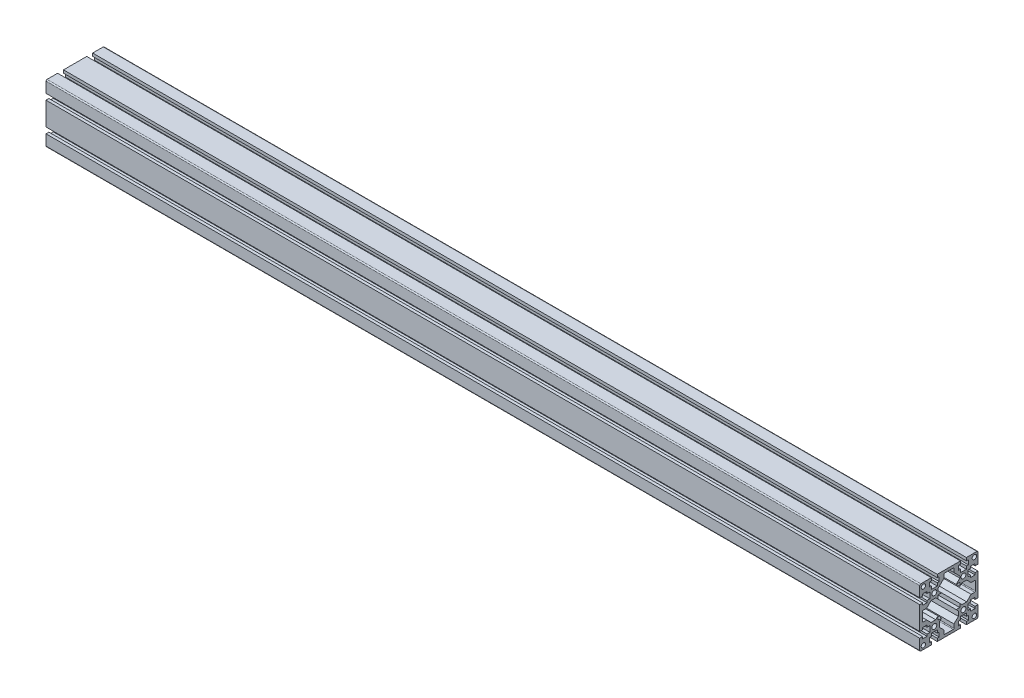
SolidWorks part; units mm, degrees
ref_plane "Front Plane" through (0, 0, 0) normal (0, 0, 1) x (1, 0, 0)
ref_plane "Top Plane" through (0, 0, 0) normal (0, 1, 0) x (1, 0, 0)
ref_plane "Right Plane" through (0, 0, 0) normal (1, 0, 0) x (0, 0, -1)
sketch "草图1" plane through (0, 0, 0) normal (0, 0, 1) x (1, 0, 0)
  line L0 (-530.3448, 0) -> (669.6552, 0)
  dimension "D1" = 1200
other "Aluminium profile 80 X 80G X R1.5(1)"
ref_plane "Plane2" through (-530.3448, 0, 0) normal (1, 0, 0) x (0, 1, 0)
sketch "Sketch1" plane through (-530.3448, 0, 0) normal (1, 0, 0) x (0, 1, 0)
  line L0 (0, 40) -> (0, 0) construction
  line L1 (0, 0) -> (40, 0) construction
  line L2 (-24.05, 40) -> (-24.05, 36)
  line L3 (-38.5, 40) -> (-24.05, 40)
  line L4 (-40, 38.5) -> (-40, 24.05)
  line L5 (-38.5, -40) -> (-24.05, -40)
  line L6 (40, 38.5) -> (40, 24.05)
  line L7 (-24.05, 36) -> (-26.75, 36)
  line L8 (-26.75, 36) -> (-26.75, 30)
  line L9 (-26.75, 30) -> (-24.05, 30)
  line L10 (-24.05, 30) -> (-24.05, 26)
  line L11 (-24.05, 26) -> (-15.95, 26)
  line L12 (-15.95, 26) -> (-15.95, 30)
  line L13 (-15.95, 30) -> (-13.25, 30)
  line L14 (-13.25, 30) -> (-13.25, 36)
  line L15 (-13.25, 36) -> (-15.95, 36)
  line L16 (-15.95, 36) -> (-15.95, 40)
  line L17 (-40, 15.95) -> (-36, 15.95)
  line L18 (-36, 15.95) -> (-36, 13.25)
  line L19 (-15.95, 40) -> (15.95, 40)
  line L20 (-20, 20) -> (-20, 40) construction
  line L21 (20, 20) -> (20, 40) construction
  line L22 (15.95, 36) -> (15.95, 40)
  line L23 (13.25, 36) -> (15.95, 36)
  line L24 (13.25, 30) -> (13.25, 36)
  line L25 (15.95, 30) -> (13.25, 30)
  line L26 (-36, 13.25) -> (-30, 13.25)
  line L27 (-30, 13.25) -> (-30, 15.95)
  line L28 (-26, 15.95) -> (-26, 24.05)
  line L29 (-26, 24.05) -> (-30, 24.05)
  line L30 (-30, 24.05) -> (-30, 26.75)
  line L31 (-30, 26.75) -> (-36, 26.75)
  line L32 (-36, 26.75) -> (-36, 24.05)
  line L33 (-36, 24.05) -> (-40, 24.05)
  line L34 (-30, 15.95) -> (-26, 15.95)
  line L35 (15.95, 26) -> (15.95, 30)
  line L36 (24.05, 26) -> (15.95, 26)
  line L37 (24.05, 30) -> (24.05, 26)
  line L38 (26.75, 30) -> (24.05, 30)
  line L39 (26.75, 36) -> (26.75, 30)
  line L40 (24.05, 36) -> (26.75, 36)
  line L41 (24.05, 40) -> (24.05, 36)
  line L42 (24.05, -40) -> (24.05, -36)
  line L43 (24.05, -36) -> (26.75, -36)
  line L44 (26.75, -36) -> (26.75, -30)
  line L45 (26.75, -30) -> (24.05, -30)
  line L46 (24.05, -30) -> (24.05, -26)
  line L47 (24.05, -26) -> (15.95, -26)
  line L48 (15.95, -26) -> (15.95, -30)
  line L49 (15.95, -30) -> (13.25, -30)
  line L50 (13.25, -30) -> (13.25, -36)
  line L51 (13.25, -36) -> (15.95, -36)
  line L52 (15.95, -36) -> (15.95, -40)
  line L53 (-15.95, -36) -> (-15.95, -40)
  line L54 (-13.25, -36) -> (-15.95, -36)
  line L55 (-13.25, -30) -> (-13.25, -36)
  line L56 (-15.95, -30) -> (-13.25, -30)
  line L57 (-15.95, -26) -> (-15.95, -30)
  line L58 (-24.05, -26) -> (-15.95, -26)
  line L59 (-24.05, -30) -> (-24.05, -26)
  line L60 (-26.75, -30) -> (-24.05, -30)
  line L61 (-26.75, -36) -> (-26.75, -30)
  line L62 (-24.05, -36) -> (-26.75, -36)
  line L63 (-24.05, -40) -> (-24.05, -36)
  line L64 (-30, -15.95) -> (-26, -15.95)
  line L65 (-36, -26.75) -> (-36, -24.05)
  line L66 (-30, -26.75) -> (-36, -26.75)
  line L67 (-30, -24.05) -> (-30, -26.75)
  line L68 (-26, -24.05) -> (-30, -24.05)
  line L69 (-26, -15.95) -> (-26, -24.05)
  line L70 (-30, -13.25) -> (-30, -15.95)
  line L71 (-36, -13.25) -> (-30, -13.25)
  line L72 (-36, -15.95) -> (-36, -13.25)
  line L73 (36, 24.05) -> (40, 24.05)
  line L74 (40, 15.95) -> (36, 15.95)
  line L75 (36, -15.95) -> (36, -13.25)
  line L76 (36, -13.25) -> (30, -13.25)
  line L77 (30, -13.25) -> (30, -15.95)
  line L78 (26, -15.95) -> (26, -24.05)
  line L79 (26, -24.05) -> (30, -24.05)
  line L80 (30, -24.05) -> (30, -26.75)
  line L81 (30, -26.75) -> (36, -26.75)
  line L82 (36, -26.75) -> (36, -24.05)
  line L83 (30, -15.95) -> (26, -15.95)
  line L84 (30, 15.95) -> (26, 15.95)
  line L85 (36, 26.75) -> (36, 24.05)
  line L86 (30, 26.75) -> (36, 26.75)
  line L87 (30, 24.05) -> (30, 26.75)
  line L88 (26, 24.05) -> (30, 24.05)
  line L89 (26, 15.95) -> (26, 24.05)
  line L90 (30, 13.25) -> (30, 15.95)
  line L91 (36, 13.25) -> (30, 13.25)
  line L92 (36, 15.95) -> (36, 13.25)
  line L93 (-36, -15.95) -> (-40, -15.95)
  line L94 (-36, -24.05) -> (-40, -24.05)
  line L95 (36, -15.95) -> (40, -15.95)
  line L96 (36, -24.05) -> (40, -24.05)
  line L97 (-13, 18) -> (-10, 15)
  line L98 (-15, 15) -> (-10, 15)
  line L99 (-15, 15) -> (-15, 10)
  line L100 (-15, -15) -> (-10, -15)
  line L101 (15, 15) -> (15, 10)
  line L102 (-18, 13) -> (-15, 10)
  line L104 (13, 18) -> (10, 15)
  line L105 (13, -18) -> (10, -15)
  line L106 (20, -15) -> (15, -10)
  line L107 (-18, -13) -> (-15, -10)
  line L108 (-13, -18) -> (-10, -15)
  line L109 (15, -10) -> (15, -15)
  line L110 (10, 15) -> (15, 15)
  line L111 (-15, -10) -> (-15, -15)
  line L112 (10, -15) -> (15, -15)
  line L113 (15, 10) -> (20, 15)
  line L235 (24.05, 40) -> (38.5, 40)
  line L249 (-40, 15.95) -> (-40, -15.95)
  line L250 (-20, 20) -> (-26, 20) construction
  line L264 (40, 15.95) -> (40, -15.95)
  line L265 (-13, 24.5) -> (-7, 30.5)
  line L266 (-7, 30.5) -> (-7, 35.5)
  line L267 (7, 35.5) -> (7, 30.5)
  line L268 (7, 30.5) -> (13, 24.5)
  line L269 (-6, -36.5) -> (6, -36.5)
  line L270 (-13, 24.5) -> (-13, 18)
  line L271 (-35.5, 7) -> (-30.5, 7)
  line L272 (-30.5, 7) -> (-24.5, 13)
  line L273 (-24.5, 13) -> (-18, 13)
  line L274 (13, 24.5) -> (13, 18)
  line L275 (-15.95, -40) -> (15.95, -40)
  line L276 (35.5, 7) -> (30.5, 7)
  line L277 (30.5, 7) -> (22.5, 15)
  line L278 (24.05, -40) -> (38.5, -40)
  line L279 (20, 15) -> (22.5, 15)
  line L333 (-13, -24.5) -> (-13, -18)
  line L336 (-13, -24.5) -> (-7, -30.5)
  line L385 (-7, -30.5) -> (-7, -35.5)
  line L386 (-36.5, 6) -> (-36.5, -6)
  line L387 (7, -35.5) -> (7, -30.5)
  line L429 (7, -30.5) -> (13, -24.5)
  line L430 (13, -24.5) -> (13, -18)
  line L494 (20, -15) -> (22.5, -15)
  line L496 (30.5, -7) -> (22.5, -15)
  line L497 (35.5, -7) -> (30.5, -7)
  line L498 (-24.5, -13) -> (-18, -13)
  line L499 (-30.5, -7) -> (-24.5, -13)
  line L500 (-35.5, -7) -> (-30.5, -7)
  line L512 (40, -24.05) -> (40, -38.5)
  line L519 (-40, -24.05) -> (-40, -38.5)
  line L520 (-6, 36.5) -> (6, 36.5)
  line L523 (36.5, 6) -> (36.5, -6)
  circle A0 centre (-20, 20) radius 3.4
  circle A2 centre (20, 20) radius 3.4
  circle A3 centre (20, -20) radius 3.4
  circle A7 centre (-20, -20) radius 3.4
  arc A8 (-38.5, 40) -> (-40, 38.5) centre (-38.5, 38.5) ccw
  arc A9 (-40, -38.5) -> (-38.5, -40) centre (-38.5, -38.5) ccw
  arc A10 (38.5, -40) -> (40, -38.5) centre (38.5, -38.5) ccw
  arc A11 (38.5, 40) -> (40, 38.5) centre (38.5, 38.5) cw
  circle A12 centre (-35, 35) radius 3
  circle A13 centre (35, 35) radius 3
  circle A14 centre (35, -35) radius 3
  arc A15 (-6, 36.5) -> (-7, 35.5) centre (-6, 35.5) ccw
  arc A16 (6, 36.5) -> (7, 35.5) centre (6, 35.5) cw
  arc A17 (-36.5, 6) -> (-35.5, 7) centre (-35.5, 6) cw
  arc A18 (-36.5, -6) -> (-35.5, -7) centre (-35.5, -6) ccw
  arc A19 (36.5, -6) -> (35.5, -7) centre (35.5, -6) cw
  arc A20 (36.5, 6) -> (35.5, 7) centre (35.5, 6) ccw
  arc A21 (6, -36.5) -> (7, -35.5) centre (6, -35.5) ccw
  arc A22 (-6, -36.5) -> (-7, -35.5) centre (-6, -35.5) cw
  point P48 (-20, 20)
  point P97 (0, 0)
  point P104 (-7, 36.5)
  point P185 (40, 40)
  point P187 (40, -40)
  point P188 (-40, -40)
  point P190 (-40, 40)
  dimension "D1" = 80
  dimension "D2" = 80
  dimension "D3" = 20
  dimension "D4" = 8.1
  dimension "D5" = 45
  dimension "D6" = 7
  dimension "D7" = 13.5
  dimension "D8" = 6
  dimension "D12" = 5
  dimension "D13" = 5
  dimension "D14" = 20
  dimension "D18" = 1
  dimension "D19" = 14
  dimension "D15" = 6.8
  dimension "D27" = 45
  dimension "D20" = 1.5
  dimension "D11" = 6
  dimension "D9" = 4
  dimension "D10" = 14
  dimension "D16" = 14
  dimension "D17" = 45
  dimension "D21" = 3.5
  dimension "D22" = 3.5
  dimension "D23" = 73
  dimension "D24" = 30
  dimension "D25" = 30
  dimension "D26" = 45
  dimension "D28" = 5
sketch "Sketch10" plane through (669.6552, 0, 0) normal (1, 0, 0) x (0, 0, -1)
  circle A0 centre (35, -35) radius 3
  circle A1 centre (-35, -35) radius 3 construction
  circle A2 centre (35, 35) radius 3 construction
  dimension "D1" = 6
  dimension "D2" = 70
  dimension "D3" = 70
extrude "Cut-Extrude1" cut sketch "Sketch10" against normal through all
